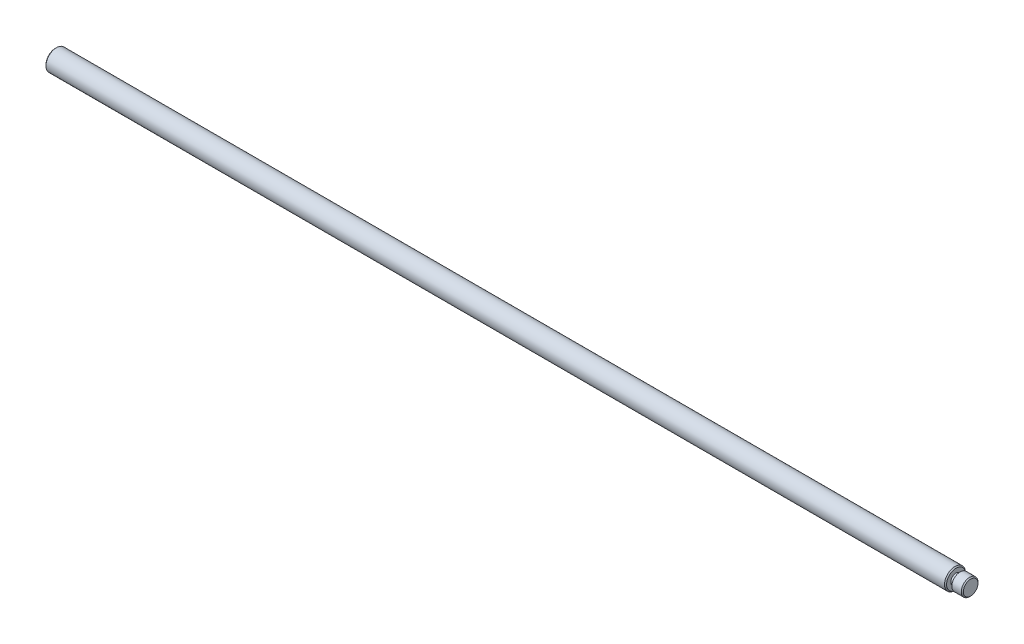
SolidWorks part; units mm, degrees
material "1060 Alloy"
ref_plane "Front Plane" through (0, 0, 0) normal (0, 0, 1) x (1, 0, 0)
ref_plane "Top Plane" through (0, 0, 0) normal (0, 1, 0) x (1, 0, 0)
ref_plane "Right Plane" through (0, 0, 0) normal (1, 0, 0) x (0, 0, -1)
other "mo"
sketch "Sketch1" plane through (0, 0, 0) normal (1, 0, 0) x (0, 0, -1)
  circle A0 centre (0, 0) radius 5
  dimension "D1" = 10
extrude "Boss-Extrude1" add sketch "Sketch1" along normal mid plane 430
sketch "Sketch2" plane through (215, 0, 0) normal (1, 0, 0) x (0, 0, -1)
  circle A0 centre (0, 0) radius 2.5
  dimension "D1" = 5
extrude "Boss-Extrude2" add sketch "Sketch2" along normal blind 2
sketch "Sketch3" plane through (217, 0, 0) normal (1, 0, 0) x (0, 0, -1)
  circle A0 centre (0, 0) radius 4
  dimension "D1" = 8
extrude "Boss-Extrude3" add sketch "Sketch3" along normal blind 5
chamfer "Chamfer1" distance 0.5 angle 45 3 edges at (222, 0, -4) (-215, 0, -5) (215, 0, -5)
